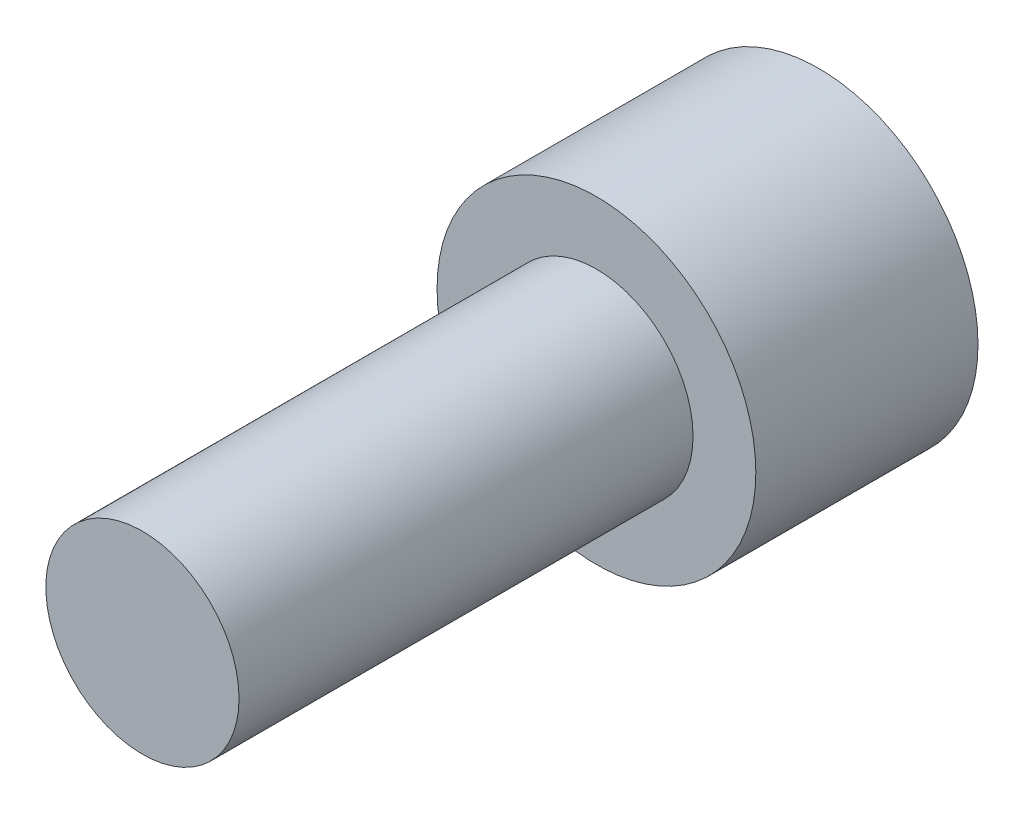
from build123d import *

# Parameters (mm, degrees)
SKETCH_1_R      = 1.65
EXTRUDE_1_DEPTH = 2.3
SKETCH_2_R      = 1
EXTRUDE_2_DEPTH = 4.7


with BuildPart() as part:
    # 草图1 → 凸台-拉伸1 (new body)
    with BuildSketch(Plane.XY):
        Circle(SKETCH_1_R)
    extrude(amount=EXTRUDE_1_DEPTH)

    # 草图2 → 凸台-拉伸2 (add)
    with BuildSketch(Plane.XY.offset(2.3)):
        Circle(SKETCH_2_R)
    extrude(amount=EXTRUDE_2_DEPTH)


solid = part.part
